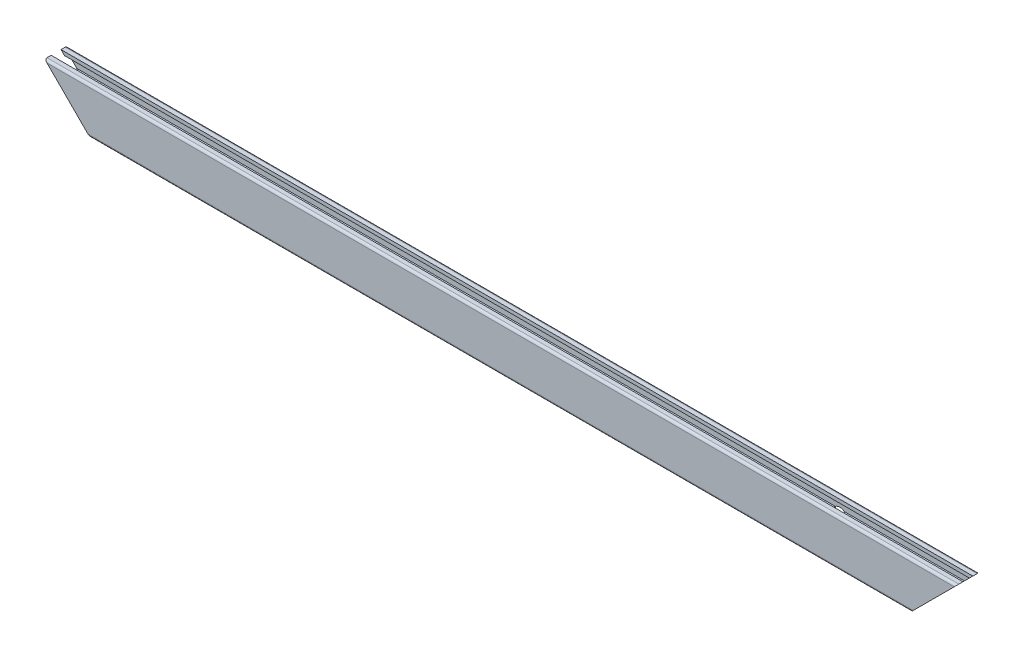
from build123d import *

# Parameters (mm, degrees)
SKETCH12_R          = 2.5
MEMBER_1_DEPTH      = 600
CUT_EXTRUDE_1_DEPTH = 301.749064836
SKETCH_7_R          = 5
CUT_EXTRUDE_2_DEPTH = 4.999


with BuildPart() as part:
    # Sketch12 → Member 1 (new body)
    with BuildSketch(Plane(origin=(-300, 0, 0), x_dir=(0, 0, -1), z_dir=(1, 0, 0))):
        with BuildLine():
            Line((-6, -15), (-3.25, -15))
            Line((-3.25, -15), (-3.25, -12.7))
            Line((-3.25, -12.7), (-5.7, -12.7))
            Line((-5.7, -12.7), (-5.7, -7))
            ThreePointArc((-5.7, -7), (0, -4.5), (5.7, -7))
            Line((5.7, -7), (5.7, -12.7))
            Line((5.7, -12.7), (3.25, -12.7))
            Line((3.25, -12.7), (3.25, -15))
            Line((3.25, -15), (6, -15))
            ThreePointArc((6, -15), (7.060660172, -14.560660172), (7.5, -13.5))
            Line((7.5, -13.5), (7.5, 13.5))
            ThreePointArc((7.5, 13.5), (7.060660172, 14.560660172), (6, 15))
            Line((6, 15), (3.25, 15))
            Line((3.25, 15), (3.25, 12.7))
            Line((3.25, 12.7), (5.7, 12.7))
            Line((5.7, 12.7), (5.7, 7))
            ThreePointArc((5.7, 7), (0, 4.5), (-5.7, 7))
            Line((-5.7, 7), (-5.7, 12.7))
            Line((-5.7, 12.7), (-3.25, 12.7))
            Line((-3.25, 12.7), (-3.25, 15))
            Line((-3.25, 15), (-6, 15))
            ThreePointArc((-6, 15), (-7.060660172, 14.560660172), (-7.5, 13.5))
            Line((-7.5, 13.5), (-7.5, -13.5))
            ThreePointArc((-7.5, -13.5), (-7.060660172, -14.560660172), (-6, -15))
        make_face()
        Circle(SKETCH12_R, mode=Mode.SUBTRACT)
    extrude(amount=MEMBER_1_DEPTH)

    # 草图4 → 切除-拉伸1 (cut, through all)
    with BuildSketch(Plane.XY.offset(7.5)):
        Polygon((-300, 15), (-270, -15), (-300, -15), align=None)
        Polygon((300, -15), (300, 15), (270, -15), align=None)
    extrude(amount=-CUT_EXTRUDE_1_DEPTH, mode=Mode.SUBTRACT)

    # 草图7 → 切除-拉伸2 (cut)
    with BuildSketch(Plane.XY.offset(-7.5)):
        with Locations(Location((210, 3, 0), (0, 0, 157.483422962))):
            Circle(SKETCH_7_R)
    extrude(amount=CUT_EXTRUDE_2_DEPTH, mode=Mode.SUBTRACT)


solid = part.part
